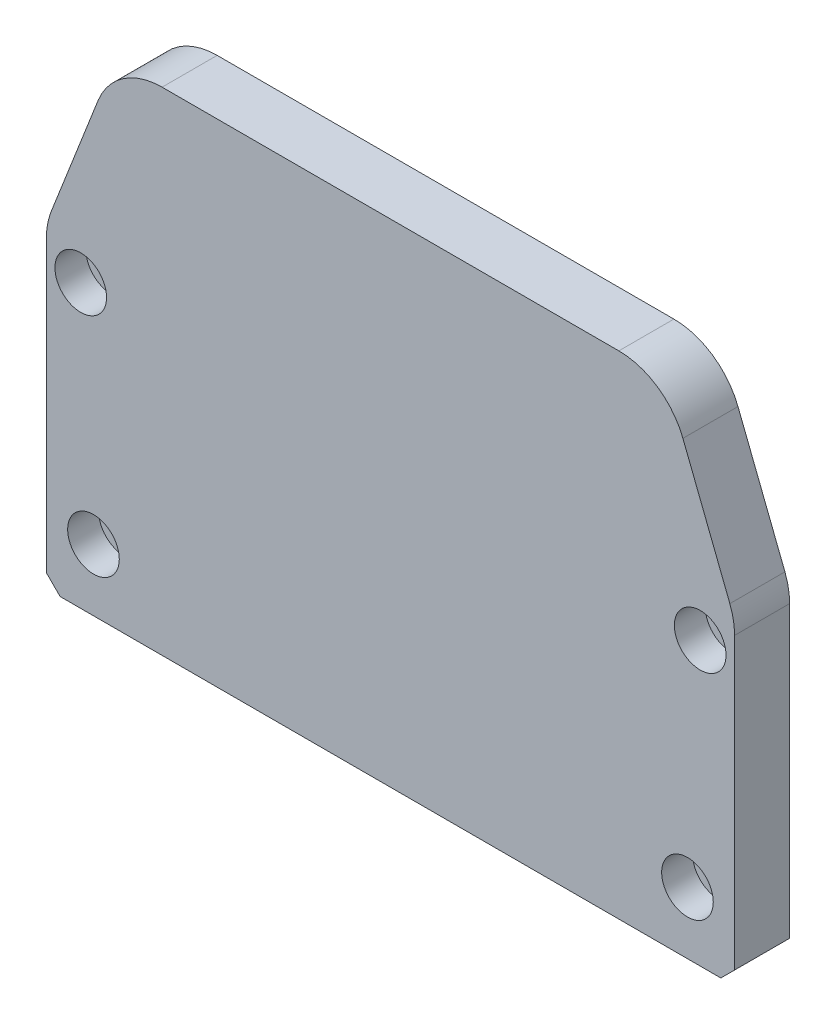
SolidWorks part; units mm, degrees
material "6061铝"
ref_plane "前视基准面" through (0, 0, 0) normal (0, 0, 1) x (1, 0, 0)
ref_plane "上视基准面" through (0, 0, 0) normal (0, 1, 0) x (1, 0, 0)
ref_plane "右视基准面" through (0, 0, 0) normal (1, 0, 0) x (0, 0, -1)
sketch "草图1" plane through (0, 0, 0) normal (0, 0, 1) x (1, 0, 0)
  line L1 (-50, -35.75) -> (50, -35.75)
  line L2 (-50, -35.75) -> (-50, 35.75)
  line L3 (-50, 35.75) -> (50, 35.75)
  line L4 (50, -35.75) -> (50, 35.75)
  line L5 (-50, -35.75) -> (50, 35.75) construction
  line L6 (-50, 35.75) -> (50, -35.75) construction
  point P0 (0, 0)
  dimension "D1" = 100
  dimension "D2" = 71.5
extrude "凸台-拉伸1" add sketch "草图1" along normal blind 8
sketch "草图3" plane through (0, 0, 0) normal (0, 0, -1) x (-1, 0, 0)
  line L0 (-50, 10.25) -> (-40, 35.75)
  line L1 (-50, -35.75) -> (-50, 35.75) construction
  line L2 (-50, 35.75) -> (50, 35.75) construction
  line L3 (-40, 35.75) -> (-50, 35.75)
  line L4 (-50, 35.75) -> (-50, 10.25)
  line L5 (50, -35.75) -> (-50, -35.75) construction
  line L6 (0, 35.75) -> (0, 59.5078) construction
  line L7 (50, 35.75) -> (50, 10.25)
  line L8 (40, 35.75) -> (50, 35.75)
  line L9 (50, 10.25) -> (40, 35.75)
  dimension "D1" = 46
  dimension "D2" = 10
extrude "切除-拉伸1" cut sketch "草图3" against normal blind 10
fillet "圆角1" radius 10 4 edges at (-50, 10.25, 4) (-40, 35.75, 4) (40, 35.75, 4) (50, 10.25, 4)
chamfer "倒角2" distance 2 angle 45 2 edges at (-50, -35.75, 4) (50, -35.75, 4)
sketch "草图4" plane through (0, 0, 0) normal (0, 0, -1) x (-1, 0, 0)
  line L0 (48, -35.75) -> (-48, -35.75) construction
  line L1 (-50, -33.75) -> (-50, 8.3593) construction
  circle A0 centre (0, 8.75) radius 17.5
  dimension "D1" = 44.5
  dimension "D2" = 35
  dimension "D3" = 50
extrude "切除-拉伸2" cut sketch "草图4" against normal blind 5
hole_wizard "打孔尺寸(%根据)内六角圆柱头螺钉的类型1" positions "草图5" profile "草图6" counterbore size "M4" standard "GB" end condition through all
sketch "草图5" plane through (0, 0, 8) normal (0, 0, 1) x (1, 0, 0)
  point P0 (-45, 5.25)
  point P3 (-43.15, -26.75)
  point P6 (45, 5.25)
  point P9 (43.15, -26.75)
sketch "草图6" plane through (-45, 5.25, 8) normal (1, 0, 0) x (0, -1, 0)
  line L0 (0, 0) -> (0, 8)
  line L1 (0, 8) -> (2.25, 8)
  line L3 (2.25, 8) -> (2.25, 4.5)
  line L4 (2.25, 4.5) -> (3.75, 4.5)
  line L5 (3.75, 4.5) -> (3.75, 0)
  line L7 (3.75, 0) -> (0, 0)
  line L11 (0, -6.35) -> (0, 107.95) construction
  dimension "通孔孔直径" = 4.5
  dimension "通孔孔深度" = 8
  dimension "柱形沉头孔直径" = 7.5
  dimension "柱形沉头孔深度" = 4.5
